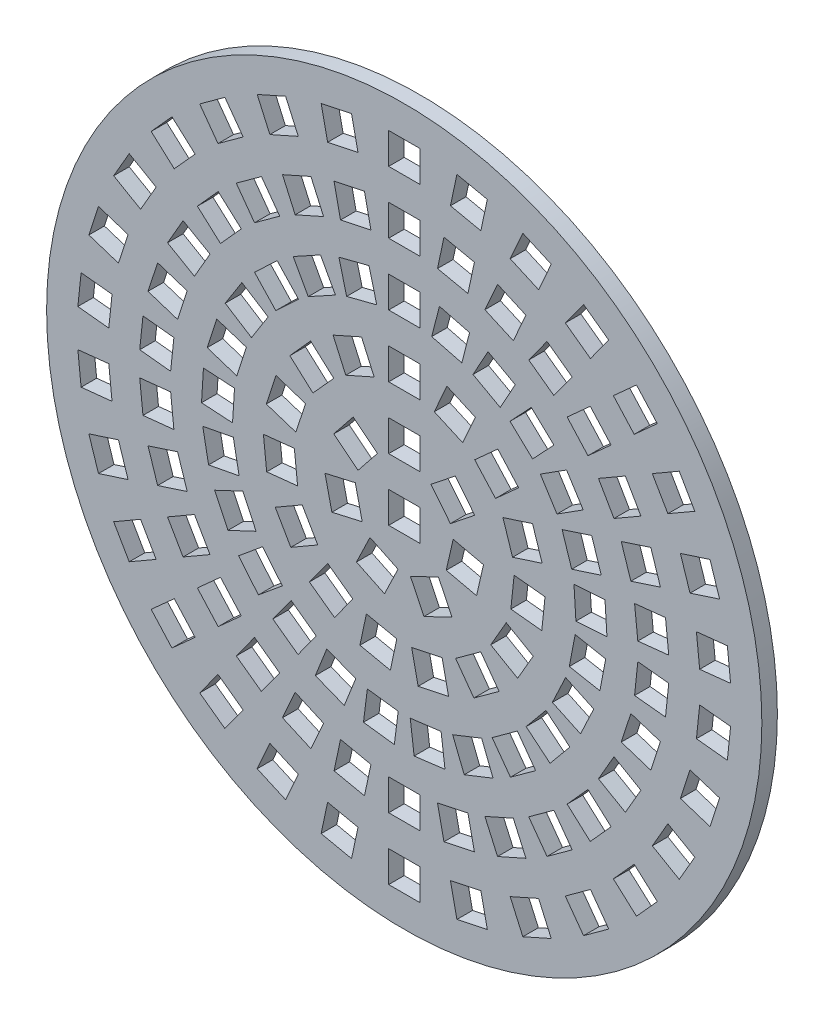
SolidWorks part; units mm, degrees
ref_plane "Front" through (0, 0, 0) normal (0, 0, 1) x (1, 0, 0)
ref_plane "Top" through (0, 0, 0) normal (0, 1, 0) x (1, 0, 0)
ref_plane "Right" through (0, 0, 0) normal (1, 0, 0) x (0, 0, -1)
sketch "Sketch1" plane through (0, 0, 0) normal (0, 0, 1) x (1, 0, 0)
  line L0 (2.9722, 18.7927) -> (4.9285, 18.3769)
  line L1 (-1, 21) -> (1, 21)
  line L2 (-1, 21) -> (-1, 19)
  line L3 (-1, 19) -> (1, 19)
  line L4 (1, 21) -> (1, 19)
  line L5 (3.388, 20.749) -> (5.3443, 20.3332)
  line L6 (5.3443, 20.3332) -> (4.9285, 18.3769)
  line L7 (6.8145, 17.7641) -> (8.6415, 16.9506)
  line L8 (7.6279, 19.5912) -> (9.455, 18.7777)
  line L9 (9.455, 18.7777) -> (8.6415, 16.9506)
  line L10 (10.3589, 15.9591) -> (11.9769, 14.7835)
  line L11 (11.5345, 17.5771) -> (13.1525, 16.4016)
  line L12 (13.1525, 16.4016) -> (11.9769, 14.7835)
  line L13 (13.4506, 13.4566) -> (14.7889, 11.9703)
  line L14 (14.9369, 14.7949) -> (16.2752, 13.3086)
  line L15 (16.2752, 13.3086) -> (14.7889, 11.9703)
  line L16 (15.9545, 10.366) -> (16.9545, 8.634)
  line L17 (17.6865, 11.366) -> (18.6865, 9.634)
  line L18 (18.6865, 9.634) -> (16.9545, 8.634)
  line L19 (17.7611, 6.8224) -> (18.3791, 4.9203)
  line L20 (19.6632, 7.4404) -> (20.2812, 5.5383)
  line L21 (20.2812, 5.5383) -> (18.3791, 4.9203)
  line L22 (18.7914, 2.9806) -> (19.0004, 0.9915)
  line L23 (20.7804, 3.1896) -> (20.9895, 1.2006)
  line L24 (20.9895, 1.2006) -> (19.0004, 0.9915)
  line L25 (19.0004, -0.9915) -> (18.7914, -2.9806)
  line L26 (20.9895, -1.2006) -> (20.7804, -3.1896)
  line L27 (20.7804, -3.1896) -> (18.7914, -2.9806)
  line L28 (18.3791, -4.9203) -> (17.7611, -6.8224)
  line L29 (20.2812, -5.5383) -> (19.6632, -7.4404)
  line L30 (19.6632, -7.4404) -> (17.7611, -6.8224)
  line L31 (16.9545, -8.634) -> (15.9545, -10.366)
  line L32 (18.6865, -9.634) -> (17.6865, -11.366)
  line L33 (17.6865, -11.366) -> (15.9545, -10.366)
  line L34 (14.7889, -11.9703) -> (13.4506, -13.4566)
  line L35 (16.2752, -13.3086) -> (14.9369, -14.7949)
  line L36 (14.9369, -14.7949) -> (13.4506, -13.4566)
  line L37 (11.9769, -14.7835) -> (10.3589, -15.9591)
  line L38 (13.1525, -16.4016) -> (11.5345, -17.5771)
  line L39 (11.5345, -17.5771) -> (10.3589, -15.9591)
  line L40 (8.6415, -16.9506) -> (6.8145, -17.7641)
  line L41 (9.455, -18.7777) -> (7.6279, -19.5912)
  line L42 (7.6279, -19.5912) -> (6.8145, -17.7641)
  line L43 (4.9285, -18.3769) -> (2.9722, -18.7927)
  line L44 (5.3443, -20.3332) -> (3.388, -20.749)
  line L45 (3.388, -20.749) -> (2.9722, -18.7927)
  line L46 (1, -19) -> (-1, -19)
  line L47 (1, -21) -> (-1, -21)
  line L48 (-1, -21) -> (-1, -19)
  line L49 (-2.9722, -18.7927) -> (-4.9285, -18.3769)
  line L50 (-3.388, -20.749) -> (-5.3443, -20.3332)
  line L51 (-5.3443, -20.3332) -> (-4.9285, -18.3769)
  line L52 (-6.8145, -17.7641) -> (-8.6415, -16.9506)
  line L53 (-7.6279, -19.5912) -> (-9.455, -18.7777)
  line L54 (-9.455, -18.7777) -> (-8.6415, -16.9506)
  line L55 (-10.3589, -15.9591) -> (-11.9769, -14.7835)
  line L56 (-11.5345, -17.5771) -> (-13.1525, -16.4016)
  line L57 (-13.1525, -16.4016) -> (-11.9769, -14.7835)
  line L58 (-13.4506, -13.4566) -> (-14.7889, -11.9703)
  line L59 (-14.9369, -14.7949) -> (-16.2752, -13.3086)
  line L60 (-16.2752, -13.3086) -> (-14.7889, -11.9703)
  line L61 (-15.9545, -10.366) -> (-16.9545, -8.634)
  line L62 (-17.6865, -11.366) -> (-18.6865, -9.634)
  line L63 (-18.6865, -9.634) -> (-16.9545, -8.634)
  line L64 (-17.7611, -6.8224) -> (-18.3791, -4.9203)
  line L65 (-19.6632, -7.4404) -> (-20.2812, -5.5383)
  line L66 (-20.2812, -5.5383) -> (-18.3791, -4.9203)
  line L67 (-18.7914, -2.9806) -> (-19.0004, -0.9915)
  line L68 (-20.7804, -3.1896) -> (-20.9895, -1.2006)
  line L69 (-20.9895, -1.2006) -> (-19.0004, -0.9915)
  line L70 (-19.0004, 0.9915) -> (-18.7914, 2.9806)
  line L71 (-20.9895, 1.2006) -> (-20.7804, 3.1896)
  line L72 (-20.7804, 3.1896) -> (-18.7914, 2.9806)
  line L73 (-18.3791, 4.9203) -> (-17.7611, 6.8224)
  line L74 (-20.2812, 5.5383) -> (-19.6632, 7.4404)
  line L75 (-19.6632, 7.4404) -> (-17.7611, 6.8224)
  line L76 (-16.9545, 8.634) -> (-15.9545, 10.366)
  line L77 (-18.6865, 9.634) -> (-17.6865, 11.366)
  line L78 (-17.6865, 11.366) -> (-15.9545, 10.366)
  line L79 (-14.7889, 11.9703) -> (-13.4506, 13.4566)
  line L80 (-16.2752, 13.3086) -> (-14.9369, 14.7949)
  line L81 (-14.9369, 14.7949) -> (-13.4506, 13.4566)
  line L82 (-11.9769, 14.7835) -> (-10.3589, 15.9591)
  line L83 (-13.1525, 16.4016) -> (-11.5345, 17.5771)
  line L84 (-11.5345, 17.5771) -> (-10.3589, 15.9591)
  line L85 (-8.6415, 16.9506) -> (-6.8145, 17.7641)
  line L86 (-9.455, 18.7777) -> (-7.6279, 19.5912)
  line L87 (-7.6279, 19.5912) -> (-6.8145, 17.7641)
  line L88 (-4.9285, 18.3769) -> (-2.9722, 18.7927)
  line L89 (-5.3443, 20.3332) -> (-3.388, 20.749)
  line L90 (-3.388, 20.749) -> (-2.9722, 18.7927)
  line L91 (3.388, 20.749) -> (2.9722, 18.7927)
  line L92 (7.6279, 19.5912) -> (6.8145, 17.7641)
  line L93 (11.5345, 17.5771) -> (10.3589, 15.9591)
  line L94 (14.9369, 14.7949) -> (13.4506, 13.4566)
  line L95 (17.6865, 11.366) -> (15.9545, 10.366)
  line L96 (19.6632, 7.4404) -> (17.7611, 6.8224)
  line L97 (20.7804, 3.1896) -> (18.7914, 2.9806)
  line L98 (20.9895, -1.2006) -> (19.0004, -0.9915)
  line L99 (20.2812, -5.5383) -> (18.3791, -4.9203)
  line L100 (18.6865, -9.634) -> (16.9545, -8.634)
  line L101 (16.2752, -13.3086) -> (14.7889, -11.9703)
  line L102 (13.1525, -16.4016) -> (11.9769, -14.7835)
  line L103 (9.455, -18.7777) -> (8.6415, -16.9506)
  line L104 (5.3443, -20.3332) -> (4.9285, -18.3769)
  line L105 (1, -21) -> (1, -19)
  line L106 (-3.388, -20.749) -> (-2.9722, -18.7927)
  line L107 (-7.6279, -19.5912) -> (-6.8145, -17.7641)
  line L108 (-11.5345, -17.5771) -> (-10.3589, -15.9591)
  line L109 (-14.9369, -14.7949) -> (-13.4506, -13.4566)
  line L110 (-17.6865, -11.366) -> (-15.9545, -10.366)
  line L111 (-19.6632, -7.4404) -> (-17.7611, -6.8224)
  line L112 (-20.7804, -3.1896) -> (-18.7914, -2.9806)
  line L113 (-20.9895, 1.2006) -> (-19.0004, 0.9915)
  line L114 (-20.2812, 5.5383) -> (-18.3791, 4.9203)
  line L115 (-18.6865, 9.634) -> (-16.9545, 8.634)
  line L116 (-16.2752, 13.3086) -> (-14.7889, 11.9703)
  line L117 (-13.1525, 16.4016) -> (-11.9769, 14.7835)
  line L118 (-9.455, 18.7777) -> (-8.6415, 16.9506)
  line L119 (-5.3443, 20.3332) -> (-4.9285, 18.3769)
  line L120 (2.5564, 16.8364) -> (2.1405, 14.8801)
  line L121 (-1, 17) -> (1, 17)
  line L122 (-1, 17) -> (-1, 15)
  line L123 (-1, 15) -> (1, 15)
  line L124 (1, 17) -> (1, 15)
  line L125 (-1, 13) -> (1, 13)
  line L126 (-1, 13) -> (-1, 11)
  line L127 (-1, 11) -> (1, 11)
  line L128 (1, 13) -> (1, 11)
  line L129 (-1, 9) -> (1, 9)
  line L130 (-1, 9) -> (-1, 7)
  line L131 (-1, 7) -> (1, 7)
  line L132 (1, 9) -> (1, 7)
  line L133 (-1, 5) -> (1, 5)
  line L134 (-1, 5) -> (-1, 3)
  line L135 (-1, 3) -> (1, 3)
  line L136 (1, 5) -> (1, 3)
  line L137 (-1, 1.0085) -> (1, 1.0085)
  line L138 (-1, 1.0085) -> (-1, -0.9915)
  line L139 (-1, -0.9915) -> (1, -0.9915)
  line L140 (1, 1.0085) -> (1, -0.9915)
  line L141 (2.5564, 16.8364) -> (4.5126, 16.4206)
  line L142 (4.5126, 16.4206) -> (4.0968, 14.4643)
  line L143 (2.1405, 14.8801) -> (4.0968, 14.4643)
  line L144 (6.001, 15.937) -> (5.1875, 14.1099)
  line L145 (6.001, 15.937) -> (7.8281, 15.1235)
  line L146 (7.8281, 15.1235) -> (7.0146, 13.2964)
  line L147 (5.1875, 14.1099) -> (7.0146, 13.2964)
  line L148 (9.1833, 14.3411) -> (8.0078, 12.723)
  line L149 (9.1833, 14.3411) -> (10.8014, 13.1655)
  line L150 (10.8014, 13.1655) -> (9.6258, 11.5475)
  line L151 (8.0078, 12.723) -> (9.6258, 11.5475)
  line L152 (11.9643, 12.1184) -> (10.478, 10.7801)
  line L153 (11.9643, 12.1184) -> (13.3026, 10.6321)
  line L154 (13.3026, 10.6321) -> (11.8163, 9.2938)
  line L155 (10.478, 10.7801) -> (11.8163, 9.2938)
  line L156 (14.2224, 9.366) -> (12.4904, 8.366)
  line L157 (14.2224, 9.366) -> (15.2224, 7.634)
  line L158 (15.2224, 7.634) -> (13.4904, 6.634)
  line L159 (12.4904, 8.366) -> (13.4904, 6.634)
  line L160 (15.8589, 6.2043) -> (13.9568, 5.5863)
  line L161 (15.8589, 6.2043) -> (16.477, 4.3022)
  line L162 (16.477, 4.3022) -> (14.5749, 3.6842)
  line L163 (13.9568, 5.5863) -> (14.5749, 3.6842)
  line L164 (16.8023, 2.7715) -> (14.8133, 2.5624)
  line L165 (16.8023, 2.7715) -> (17.0114, 0.7825)
  line L166 (17.0114, 0.7825) -> (15.0224, 0.5734)
  line L167 (14.8133, 2.5624) -> (15.0224, 0.5734)
  line L168 (17.0114, -0.7825) -> (15.0224, -0.5734)
  line L169 (17.0114, -0.7825) -> (16.8023, -2.7715)
  line L170 (16.8023, -2.7715) -> (14.8133, -2.5624)
  line L171 (15.0224, -0.5734) -> (14.8133, -2.5624)
  line L172 (16.477, -4.3022) -> (14.5749, -3.6842)
  line L173 (16.477, -4.3022) -> (15.8589, -6.2043)
  line L174 (15.8589, -6.2043) -> (13.9568, -5.5863)
  line L175 (14.5749, -3.6842) -> (13.9568, -5.5863)
  line L176 (15.2224, -7.634) -> (13.4904, -6.634)
  line L177 (15.2224, -7.634) -> (14.2224, -9.366)
  line L178 (14.2224, -9.366) -> (12.4904, -8.366)
  line L179 (13.4904, -6.634) -> (12.4904, -8.366)
  line L180 (13.3026, -10.6321) -> (11.8163, -9.2938)
  line L181 (13.3026, -10.6321) -> (11.9643, -12.1184)
  line L182 (11.9643, -12.1184) -> (10.478, -10.7801)
  line L183 (11.8163, -9.2938) -> (10.478, -10.7801)
  line L184 (10.8014, -13.1655) -> (9.6258, -11.5475)
  line L185 (10.8014, -13.1655) -> (9.1833, -14.3411)
  line L186 (9.1833, -14.3411) -> (8.0078, -12.723)
  line L187 (9.6258, -11.5475) -> (8.0078, -12.723)
  line L188 (7.8281, -15.1235) -> (7.0146, -13.2964)
  line L189 (7.8281, -15.1235) -> (6.001, -15.937)
  line L190 (6.001, -15.937) -> (5.1875, -14.1099)
  line L191 (7.0146, -13.2964) -> (5.1875, -14.1099)
  line L192 (4.5126, -16.4206) -> (4.0968, -14.4643)
  line L193 (4.5126, -16.4206) -> (2.5564, -16.8364)
  line L194 (2.5564, -16.8364) -> (2.1405, -14.8801)
  line L195 (4.0968, -14.4643) -> (2.1405, -14.8801)
  line L196 (1, -17) -> (1, -15)
  line L197 (1, -17) -> (-1, -17)
  line L198 (-1, -17) -> (-1, -15)
  line L199 (1, -15) -> (-1, -15)
  line L200 (-2.5564, -16.8364) -> (-2.1405, -14.8801)
  line L201 (-2.5564, -16.8364) -> (-4.5126, -16.4206)
  line L202 (-4.5126, -16.4206) -> (-4.0968, -14.4643)
  line L203 (-2.1405, -14.8801) -> (-4.0968, -14.4643)
  line L204 (-6.001, -15.937) -> (-5.1875, -14.1099)
  line L205 (-6.001, -15.937) -> (-7.8281, -15.1235)
  line L206 (-7.8281, -15.1235) -> (-7.0146, -13.2964)
  line L207 (-5.1875, -14.1099) -> (-7.0146, -13.2964)
  line L208 (-9.1833, -14.3411) -> (-8.0078, -12.723)
  line L209 (-9.1833, -14.3411) -> (-10.8014, -13.1655)
  line L210 (-10.8014, -13.1655) -> (-9.6258, -11.5475)
  line L211 (-8.0078, -12.723) -> (-9.6258, -11.5475)
  line L212 (-11.9643, -12.1184) -> (-10.478, -10.7801)
  line L213 (-11.9643, -12.1184) -> (-13.3026, -10.6321)
  line L214 (-13.3026, -10.6321) -> (-11.8163, -9.2938)
  line L215 (-10.478, -10.7801) -> (-11.8163, -9.2938)
  line L216 (-14.2224, -9.366) -> (-12.4904, -8.366)
  line L217 (-14.2224, -9.366) -> (-15.2224, -7.634)
  line L218 (-15.2224, -7.634) -> (-13.4904, -6.634)
  line L219 (-12.4904, -8.366) -> (-13.4904, -6.634)
  line L220 (-15.8589, -6.2043) -> (-13.9568, -5.5863)
  line L221 (-15.8589, -6.2043) -> (-16.477, -4.3022)
  line L222 (-16.477, -4.3022) -> (-14.5749, -3.6842)
  line L223 (-13.9568, -5.5863) -> (-14.5749, -3.6842)
  line L224 (-16.8023, -2.7715) -> (-14.8133, -2.5624)
  line L225 (-16.8023, -2.7715) -> (-17.0114, -0.7825)
  line L226 (-17.0114, -0.7825) -> (-15.0224, -0.5734)
  line L227 (-14.8133, -2.5624) -> (-15.0224, -0.5734)
  line L228 (-17.0114, 0.7825) -> (-15.0224, 0.5734)
  line L229 (-17.0114, 0.7825) -> (-16.8023, 2.7715)
  line L230 (-16.8023, 2.7715) -> (-14.8133, 2.5624)
  line L231 (-15.0224, 0.5734) -> (-14.8133, 2.5624)
  line L232 (-16.477, 4.3022) -> (-14.5749, 3.6842)
  line L233 (-16.477, 4.3022) -> (-15.8589, 6.2043)
  line L234 (-15.8589, 6.2043) -> (-13.9568, 5.5863)
  line L235 (-14.5749, 3.6842) -> (-13.9568, 5.5863)
  line L236 (-15.2224, 7.634) -> (-13.4904, 6.634)
  line L237 (-15.2224, 7.634) -> (-14.2224, 9.366)
  line L238 (-14.2224, 9.366) -> (-12.4904, 8.366)
  line L239 (-13.4904, 6.634) -> (-12.4904, 8.366)
  line L240 (-13.3026, 10.6321) -> (-11.8163, 9.2938)
  line L241 (-13.3026, 10.6321) -> (-11.9643, 12.1184)
  line L242 (-11.9643, 12.1184) -> (-10.478, 10.7801)
  line L243 (-11.8163, 9.2938) -> (-10.478, 10.7801)
  line L244 (-10.8014, 13.1655) -> (-9.6258, 11.5475)
  line L245 (-10.8014, 13.1655) -> (-9.1833, 14.3411)
  line L246 (-9.1833, 14.3411) -> (-8.0078, 12.723)
  line L247 (-9.6258, 11.5475) -> (-8.0078, 12.723)
  line L248 (-7.8281, 15.1235) -> (-7.0146, 13.2964)
  line L249 (-7.8281, 15.1235) -> (-6.001, 15.937)
  line L250 (-6.001, 15.937) -> (-5.1875, 14.1099)
  line L251 (-7.0146, 13.2964) -> (-5.1875, 14.1099)
  line L252 (-4.5126, 16.4206) -> (-4.0968, 14.4643)
  line L253 (-4.5126, 16.4206) -> (-2.5564, 16.8364)
  line L254 (-2.5564, 16.8364) -> (-2.1405, 14.8801)
  line L255 (-4.0968, 14.4643) -> (-2.1405, 14.8801)
  line L256 (2.2644, 12.8403) -> (1.767, 10.9031)
  line L257 (2.2644, 12.8403) -> (4.2016, 12.3429)
  line L258 (4.2016, 12.3429) -> (3.7042, 10.4057)
  line L259 (1.767, 10.9031) -> (3.7042, 10.4057)
  line L260 (5.3865, 11.8737) -> (4.423, 10.1211)
  line L261 (5.3865, 11.8737) -> (7.1391, 10.9102)
  line L262 (7.1391, 10.9102) -> (6.1756, 9.1576)
  line L263 (4.423, 10.1211) -> (6.1756, 9.1576)
  line L264 (8.1701, 10.1611) -> (6.801, 8.7032)
  line L265 (8.1701, 10.1611) -> (9.6281, 8.792)
  line L266 (9.6281, 8.792) -> (8.259, 7.3341)
  line L267 (6.801, 8.7032) -> (8.259, 7.3341)
  line L268 (10.4404, 7.8101) -> (8.7518, 6.7384)
  line L269 (10.4404, 7.8101) -> (11.5121, 6.1214)
  line L270 (11.5121, 6.1214) -> (9.8234, 5.0498)
  line L271 (8.7518, 6.7384) -> (9.8234, 5.0498)
  line L272 (12.0547, 4.9683) -> (10.1526, 4.3502)
  line L273 (12.0547, 4.9683) -> (12.6728, 3.0662)
  line L274 (12.6728, 3.0662) -> (10.7706, 2.4481)
  line L275 (10.1526, 4.3502) -> (10.7706, 2.4481)
  line L276 (12.9116, 1.8143) -> (10.9155, 1.6887)
  line L277 (12.9116, 1.8143) -> (13.0371, -0.1817)
  line L278 (13.0371, -0.1817) -> (11.0411, -0.3073)
  line L279 (10.9155, 1.6887) -> (11.0411, -0.3073)
  line L280 (12.9571, -1.4537) -> (10.9925, -1.0789)
  line L281 (12.9571, -1.4537) -> (12.5824, -3.4182)
  line L282 (12.5824, -3.4182) -> (10.6178, -3.0435)
  line L283 (10.9925, -1.0789) -> (10.6178, -3.0435)
  line L284 (12.1885, -4.6303) -> (10.3789, -3.7787)
  line L285 (12.1885, -4.6303) -> (11.337, -6.44)
  line L286 (11.337, -6.44) -> (9.5273, -5.5884)
  line L287 (10.3789, -3.7787) -> (9.5273, -5.5884)
  line L288 (10.6541, -7.516) -> (9.1131, -6.2412)
  line L289 (10.6541, -7.516) -> (9.3792, -9.057)
  line L290 (9.3792, -9.057) -> (7.8382, -7.7822)
  line L291 (9.1131, -6.2412) -> (7.8382, -7.7822)
  line L292 (8.4502, -9.9294) -> (7.2747, -8.3114)
  line L293 (8.4502, -9.9294) -> (6.8322, -11.105)
  line L294 (6.8322, -11.105) -> (5.6566, -9.487)
  line L295 (7.2747, -8.3114) -> (5.6566, -9.487)
  line L296 (5.7154, -11.719) -> (4.9791, -9.8594)
  line L297 (5.7154, -11.719) -> (3.8558, -12.4552)
  line L298 (3.8558, -12.4552) -> (3.1196, -10.5957)
  line L299 (4.9791, -9.8594) -> (3.1196, -10.5957)
  line L300 (2.6214, -12.7722) -> (2.3708, -10.7879)
  line L301 (2.6214, -12.7722) -> (0.6372, -13.0228)
  line L302 (0.6372, -13.0228) -> (0.3866, -11.0386)
  line L303 (2.3708, -10.7879) -> (0.3866, -11.0386)
  line L304 (-0.6372, -13.0228) -> (-0.3866, -11.0386)
  line L305 (-0.6372, -13.0228) -> (-2.6214, -12.7722)
  line L306 (-2.6214, -12.7722) -> (-2.3708, -10.7879)
  line L307 (-0.3866, -11.0386) -> (-2.3708, -10.7879)
  line L308 (-3.8558, -12.4552) -> (-3.1196, -10.5957)
  line L309 (-3.8558, -12.4552) -> (-5.7154, -11.719)
  line L310 (-5.7154, -11.719) -> (-4.9791, -9.8594)
  line L311 (-3.1196, -10.5957) -> (-4.9791, -9.8594)
  line L312 (-6.8322, -11.105) -> (-5.6566, -9.487)
  line L313 (-6.8322, -11.105) -> (-8.4502, -9.9294)
  line L314 (-8.4502, -9.9294) -> (-7.2747, -8.3114)
  line L315 (-5.6566, -9.487) -> (-7.2747, -8.3114)
  line L316 (-9.3792, -9.057) -> (-7.8382, -7.7822)
  line L317 (-9.3792, -9.057) -> (-10.6541, -7.516)
  line L318 (-10.6541, -7.516) -> (-9.1131, -6.2412)
  line L319 (-7.8382, -7.7822) -> (-9.1131, -6.2412)
  line L320 (-11.337, -6.44) -> (-9.5273, -5.5884)
  line L321 (-11.337, -6.44) -> (-12.1885, -4.6303)
  line L322 (-12.1885, -4.6303) -> (-10.3789, -3.7787)
  line L323 (-9.5273, -5.5884) -> (-10.3789, -3.7787)
  line L324 (-12.5824, -3.4182) -> (-10.6178, -3.0435)
  line L325 (-12.5824, -3.4182) -> (-12.9571, -1.4537)
  line L326 (-12.9571, -1.4537) -> (-10.9925, -1.0789)
  line L327 (-10.6178, -3.0435) -> (-10.9925, -1.0789)
  line L328 (-13.0371, -0.1817) -> (-11.0411, -0.3073)
  line L329 (-13.0371, -0.1817) -> (-12.9116, 1.8143)
  line L330 (-12.9116, 1.8143) -> (-10.9155, 1.6887)
  line L331 (-11.0411, -0.3073) -> (-10.9155, 1.6887)
  line L332 (-12.6728, 3.0662) -> (-10.7706, 2.4481)
  line L333 (-12.6728, 3.0662) -> (-12.0547, 4.9683)
  line L334 (-12.0547, 4.9683) -> (-10.1526, 4.3502)
  line L335 (-10.7706, 2.4481) -> (-10.1526, 4.3502)
  line L336 (-11.5121, 6.1214) -> (-9.8234, 5.0498)
  line L337 (-11.5121, 6.1214) -> (-10.4404, 7.8101)
  line L338 (-10.4404, 7.8101) -> (-8.7518, 6.7384)
  line L339 (-9.8234, 5.0498) -> (-8.7518, 6.7384)
  line L340 (-9.6281, 8.792) -> (-8.259, 7.3341)
  line L341 (-9.6281, 8.792) -> (-8.1701, 10.1611)
  line L342 (-8.1701, 10.1611) -> (-6.801, 8.7032)
  line L343 (-8.259, 7.3341) -> (-6.801, 8.7032)
  line L344 (-7.1391, 10.9102) -> (-6.1756, 9.1576)
  line L345 (-7.1391, 10.9102) -> (-5.3865, 11.8737)
  line L346 (-5.3865, 11.8737) -> (-4.423, 10.1211)
  line L347 (-6.1756, 9.1576) -> (-4.423, 10.1211)
  line L348 (-4.2016, 12.3429) -> (-3.7042, 10.4057)
  line L349 (-4.2016, 12.3429) -> (-2.2644, 12.8403)
  line L350 (-2.2644, 12.8403) -> (-1.767, 10.9031)
  line L351 (-3.7042, 10.4057) -> (-1.767, 10.9031)
  line L364 (2.7471, 8.6286) -> (1.9336, 6.8016)
  line L365 (4.5742, 7.8152) -> (3.7607, 5.9881)
  line L366 (2.7471, 8.6286) -> (4.5742, 7.8152)
  line L367 (1.9336, 6.8016) -> (3.7607, 5.9881)
  line L368 (6.0192, 6.7653) -> (4.5329, 5.4271)
  line L369 (7.3574, 5.279) -> (5.8711, 3.9408)
  line L370 (6.0192, 6.7653) -> (7.3574, 5.279)
  line L371 (4.5329, 5.4271) -> (5.8711, 3.9408)
  line L372 (8.2505, 3.7322) -> (6.3484, 3.1142)
  line L373 (8.8685, 1.8301) -> (6.9664, 1.2121)
  line L374 (8.2505, 3.7322) -> (8.8685, 1.8301)
  line L375 (6.3484, 3.1142) -> (6.9664, 1.2121)
  line L376 (9.0552, 0.0538) -> (7.0662, 0.2628)
  line L377 (8.8462, -1.9353) -> (6.8571, -1.7262)
  line L378 (9.0552, 0.0538) -> (8.8462, -1.9353)
  line L379 (7.0662, 0.2628) -> (6.8571, -1.7262)
  line L380 (8.2942, -3.634) -> (6.5622, -2.634)
  line L381 (7.2942, -5.366) -> (5.5622, -4.366)
  line L382 (8.2942, -3.634) -> (7.2942, -5.366)
  line L383 (6.5622, -2.634) -> (5.5622, -4.366)
  line L384 (6.0991, -6.6934) -> (4.9235, -5.0753)
  line L385 (4.4811, -7.8689) -> (3.3055, -6.2509)
  line L386 (6.0991, -6.6934) -> (4.4811, -7.8689)
  line L387 (4.9235, -5.0753) -> (3.3055, -6.2509)
  line L388 (2.8494, -8.5954) -> (2.4335, -6.6391)
  line L389 (0.8931, -9.0112) -> (0.4772, -7.0549)
  line L390 (2.8494, -8.5954) -> (0.8931, -9.0112)
  line L391 (2.4335, -6.6391) -> (0.4772, -7.0549)
  line L392 (-0.8931, -9.0112) -> (-0.4772, -7.0549)
  line L393 (-2.8494, -8.5954) -> (-2.4335, -6.6391)
  line L394 (-0.8931, -9.0112) -> (-2.8494, -8.5954)
  line L395 (-0.4772, -7.0549) -> (-2.4335, -6.6391)
  line L396 (-4.4811, -7.8689) -> (-3.3055, -6.2509)
  line L397 (-6.0991, -6.6934) -> (-4.9235, -5.0753)
  line L398 (-4.4811, -7.8689) -> (-6.0991, -6.6934)
  line L399 (-3.3055, -6.2509) -> (-4.9235, -5.0753)
  line L400 (-7.2942, -5.366) -> (-5.5622, -4.366)
  line L401 (-8.2942, -3.634) -> (-6.5622, -2.634)
  line L402 (-7.2942, -5.366) -> (-8.2942, -3.634)
  line L403 (-5.5622, -4.366) -> (-6.5622, -2.634)
  line L404 (-8.8462, -1.9353) -> (-6.8571, -1.7262)
  line L405 (-9.0552, 0.0538) -> (-7.0662, 0.2628)
  line L406 (-8.8462, -1.9353) -> (-9.0552, 0.0538)
  line L407 (-6.8571, -1.7262) -> (-7.0662, 0.2628)
  line L408 (-8.8685, 1.8301) -> (-6.9664, 1.2121)
  line L409 (-8.2505, 3.7322) -> (-6.3484, 3.1142)
  line L410 (-8.8685, 1.8301) -> (-8.2505, 3.7322)
  line L411 (-6.9664, 1.2121) -> (-6.3484, 3.1142)
  line L412 (-7.3574, 5.279) -> (-5.8711, 3.9408)
  line L413 (-6.0192, 6.7653) -> (-4.5329, 5.4271)
  line L414 (-7.3574, 5.279) -> (-6.0192, 6.7653)
  line L415 (-5.8711, 3.9408) -> (-4.5329, 5.4271)
  line L416 (-4.5742, 7.8152) -> (-3.7607, 5.9881)
  line L417 (-2.7471, 8.6286) -> (-1.9336, 6.8016)
  line L418 (-4.5742, 7.8152) -> (-2.7471, 8.6286)
  line L419 (-3.7607, 5.9881) -> (-1.9336, 6.8016)
  line L420 (3.2857, 3.8993) -> (1.722, 2.6523)
  line L421 (3.2857, 3.8993) -> (4.5326, 2.3356)
  line L422 (4.5326, 2.3356) -> (2.969, 1.0886)
  line L423 (1.722, 2.6523) -> (2.969, 1.0886)
  line L424 (5.0972, -0.1377) -> (3.1473, 0.3074)
  line L425 (5.0972, -0.1377) -> (4.6521, -2.0875)
  line L426 (4.6521, -2.0875) -> (2.7023, -1.6425)
  line L427 (3.1473, 0.3074) -> (2.7023, -1.6425)
  line L428 (3.0704, -4.071) -> (2.2026, -2.269)
  line L429 (3.0704, -4.071) -> (1.2684, -4.9387)
  line L430 (1.2684, -4.9387) -> (0.4007, -3.1368)
  line L431 (2.2026, -2.269) -> (0.4007, -3.1368)
  line L432 (-1.2684, -4.9387) -> (-0.4007, -3.1368)
  line L433 (-1.2684, -4.9387) -> (-3.0704, -4.071)
  line L434 (-3.0704, -4.071) -> (-2.2026, -2.269)
  line L435 (-0.4007, -3.1368) -> (-2.2026, -2.269)
  line L436 (-4.6521, -2.0875) -> (-2.7023, -1.6425)
  line L437 (-4.6521, -2.0875) -> (-5.0972, -0.1377)
  line L438 (-5.0972, -0.1377) -> (-3.1473, 0.3074)
  line L439 (-2.7023, -1.6425) -> (-3.1473, 0.3074)
  line L440 (-4.5326, 2.3356) -> (-2.969, 1.0886)
  line L441 (-4.5326, 2.3356) -> (-3.2857, 3.8993)
  line L442 (-3.2857, 3.8993) -> (-1.722, 2.6523)
  line L443 (-2.969, 1.0886) -> (-1.722, 2.6523)
  circle A0 centre (0, 0) radius 23
  point P125 (0, 0)
  point P185 (0, 0)
  point P263 (0, 0)
  point P360 (0, 0)
  point P374 (0, 0)
  point P430 (0, 0)
  point P455 (0, 0)
  dimension "D1" = 46
  dimension "D2" = 2
  dimension "D3" = 2
  dimension "D4" = 1
  dimension "D5" = 21
  dimension "D8" = 2
  dimension "D9" = 2
  dimension "D10" = 2
  dimension "D11" = 2
  dimension "D12" = 2
  dimension "D13" = 2
  dimension "D14" = 2
  dimension "D15" = 2
  dimension "D16" = 2
  dimension "D17" = 2
  dimension "D18" = 2
  dimension "D19" = 2
  dimension "D20" = 2
  dimension "D21" = 1
  dimension "D6" = 30
  dimension "D7" = 30
  dimension "D22" = 30
  dimension "D23" = 25
  dimension "D25" = 15
  dimension "D26" = 7
extrude "Boss-Extrude1" add sketch "Sketch1" along normal blind 1
